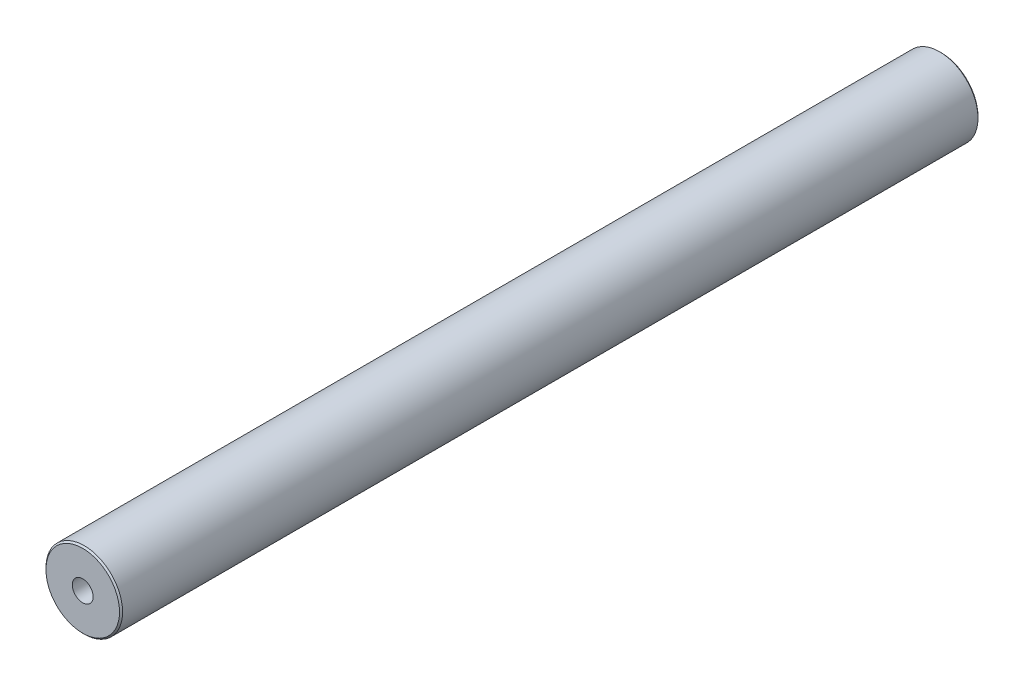
from build123d import *

# Parameters (mm, degrees)
SKETCH_1_R             = 12.5
EXTRUDE_1_DEPTH        = 280
HOLE_WIZARD_M8_1_D     = 6.8
HOLE_WIZARD_M8_1_DEPTH = 22.25
HOLE_WIZARD_M8_1_TIP   = 2.042926105
HOLE_WIZARD_M8_2_D     = 6.8
HOLE_WIZARD_M8_2_DEPTH = 22.25
HOLE_WIZARD_M8_2_TIP   = 2.042926105
CHAMFER_1_SIZE         = 0.5


with BuildPart() as part:
    # 草图1 → 凸台-拉伸1 (new body)
    with BuildSketch(Plane.XY):
        Circle(SKETCH_1_R)
    extrude(amount=EXTRUDE_1_DEPTH)

    # M8 螺纹孔1
    with Locations(Plane.XY.offset(280)):
        with Locations((0, 0)):
            Hole(HOLE_WIZARD_M8_1_D / 2, depth=HOLE_WIZARD_M8_1_DEPTH)
            with Locations((0, 0, -(HOLE_WIZARD_M8_1_DEPTH + HOLE_WIZARD_M8_1_TIP / 2))):  # 118° drill point
                Cone(0, HOLE_WIZARD_M8_1_D / 2, HOLE_WIZARD_M8_1_TIP, mode=Mode.SUBTRACT)

    # M8 螺纹孔2
    with Locations(Plane(origin=(0, 0, 0), x_dir=(-1, 0, 0), z_dir=(0, 0, -1))):
        with Locations((0, 0)):
            Hole(HOLE_WIZARD_M8_2_D / 2, depth=HOLE_WIZARD_M8_2_DEPTH)
            with Locations((0, 0, -(HOLE_WIZARD_M8_2_DEPTH + HOLE_WIZARD_M8_2_TIP / 2))):  # 118° drill point
                Cone(0, HOLE_WIZARD_M8_2_D / 2, HOLE_WIZARD_M8_2_TIP, mode=Mode.SUBTRACT)

    # 倒角1
    chamfer_1_edges = [part.edges().sort_by_distance(p)[0] for p in [
        (-12.5, 0, 0),
        (-12.5, 0, 280),
    ]]
    chamfer(chamfer_1_edges, length=CHAMFER_1_SIZE)


solid = part.part
